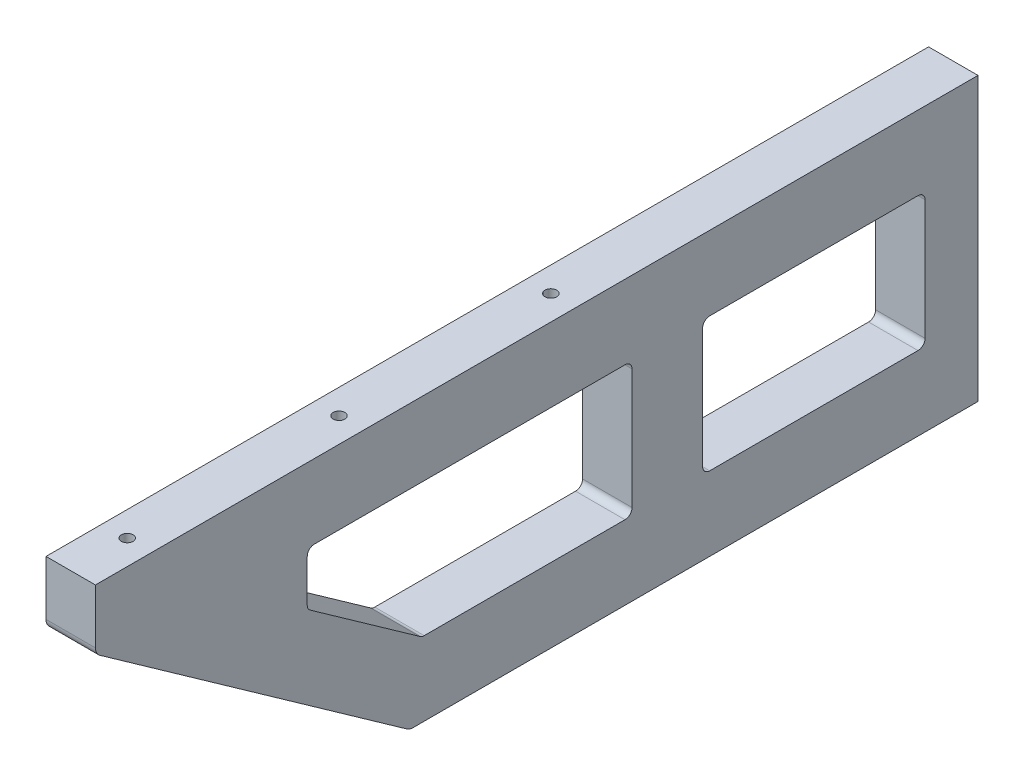
from build123d import *

# Parameters (mm, degrees)
BOSS_EXTRUDE1_DEPTH   = 7
SKETCH4_W             = 63
SKETCH4_H             = 38
CUT_EXTRUDE1_DEPTH    = 323.811382974
FILLET1_R             = 2
CUT_EXTRUDE2_DEPTH    = 323.811382974
FILLET2_R             = 2
M5_TAPPED_HOLE1_D     = 4.2
M5_TAPPED_HOLE1_DEPTH = 14
M5_TAPPED_HOLE1_TIP   = 1.2618073
M4_TAPPED_HOLE1_D     = 3.3
M4_TAPPED_HOLE1_DEPTH = 11.5
M4_TAPPED_HOLE1_TIP   = 0.991420021
FILLET3_R             = 3


with BuildPart() as part:
    # Sketch3 → Boss-Extrude1 (new, symmetric)
    with BuildSketch(Plane(origin=(50, 414.547428979, -101), x_dir=(0, 0, -1), z_dir=(-1, 0, 0))):
        Polygon((-101, 210.80448069), (-101, 290.80448069), (-262, 290.80448069), (-351, 227.80448069), (-351, 210.80448069), align=None)
    extrude(amount=BOSS_EXTRUDE1_DEPTH, both=True)

    # Sketch4 → Cut-Extrude1 (cut, through all)
    with BuildSketch(Plane(origin=(57, 0, 0), x_dir=(0, 0, -1), z_dir=(1, 0, 0))):
        with Locations((-46.5, 163.74294829)):
            Rectangle(SKETCH4_W, SKETCH4_H)
    extrude(amount=-CUT_EXTRUDE1_DEPTH, mode=Mode.SUBTRACT)

    # Fillet1
    fillet1_edges = [part.edges().sort_by_distance(p)[0] for p in [
        (50, 182.74294829, 15),
        (50, 144.74294829, 15),
        (50, 144.74294829, 78),
        (50, 182.74294829, 78),
    ]]
    fillet(fillet1_edges, radius=FILLET1_R)

    # Sketch5 → Cut-Extrude2 (cut, through all)
    with BuildSketch(Plane(origin=(57, 0, 0), x_dir=(0, 0, -1), z_dir=(1, 0, 0))):
        Polygon((-98, 144.74294829), (-157.507936508, 144.74294829), (-190, 167.74294829), (-190, 182.74294829), (-98, 182.74294829), align=None)
    extrude(amount=-CUT_EXTRUDE2_DEPTH, mode=Mode.SUBTRACT)

    # Fillet2
    fillet2_edges = [part.edges().sort_by_distance(p)[0] for p in [
        (50, 182.74294829, 98),
        (50, 144.74294829, 98),
        (50, 144.74294829, 157.507936508),
        (50, 167.74294829, 190),
        (50, 182.74294829, 190),
    ]]
    fillet(fillet2_edges, radius=FILLET2_R)

    # M5 Tapped Hole1
    with Locations(Plane(origin=(0, 0, 0), x_dir=(-1, 0, 0), z_dir=(0, 0, -1))):
        with Locations((-50.5, 188.74294829), (-50, 138.745448352)):
            Hole(M5_TAPPED_HOLE1_D / 2, depth=M5_TAPPED_HOLE1_DEPTH)
            with Locations((0, 0, -(M5_TAPPED_HOLE1_DEPTH + M5_TAPPED_HOLE1_TIP / 2))):  # 118° drill point
                Cone(0, M5_TAPPED_HOLE1_D / 2, M5_TAPPED_HOLE1_TIP, mode=Mode.SUBTRACT)

    # M4 Tapped Hole1
    with Locations(Plane(origin=(0, 203.74294829, 0), x_dir=(1, 0, 0), z_dir=(0, 1, 0))):
        with Locations((50, -114), (50, -174), (50, -234)):
            Hole(M4_TAPPED_HOLE1_D / 2, depth=M4_TAPPED_HOLE1_DEPTH)
            with Locations((0, 0, -(M4_TAPPED_HOLE1_DEPTH + M4_TAPPED_HOLE1_TIP / 2))):  # 118° drill point
                Cone(0, M4_TAPPED_HOLE1_D / 2, M4_TAPPED_HOLE1_TIP, mode=Mode.SUBTRACT)

    # Fillet3
    fillet3_edges = [part.edges().sort_by_distance(p)[0] for p in [
        (50, 186.74294829, 250),
        (50, 123.74294829, 161),
    ]]
    fillet(fillet3_edges, radius=FILLET3_R)


solid = part.part
